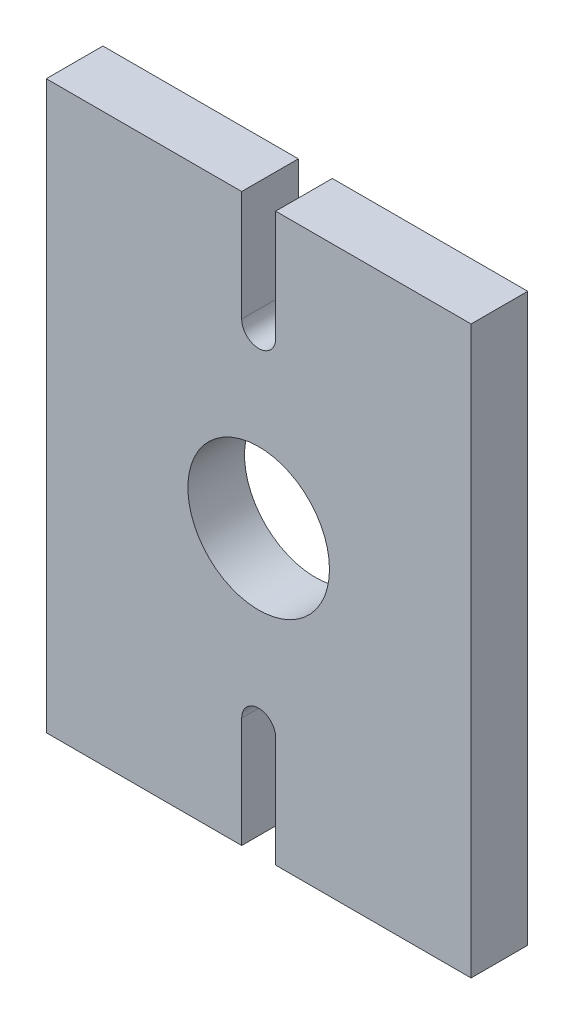
SolidWorks part; units mm, degrees
material "Q235"
ref_plane "Front Plane" through (0, 0, 0) normal (0, 0, 1) x (1, 0, 0)
ref_plane "Top Plane" through (0, 0, 0) normal (0, 1, 0) x (1, 0, 0)
ref_plane "Right Plane" through (0, 0, 0) normal (1, 0, 0) x (0, 0, -1)
sketch "Sketch1" plane through (0, 0, 0) normal (0, 0, 1) x (1, 0, 0)
  line L0 (75, 200) -> (75, 0) construction
  line L1 (0, 0) -> (69, 0)
  line L2 (0, 0) -> (0, 200)
  line L3 (0, 200) -> (69, 200)
  line L4 (150, 0) -> (150, 200)
  line L5 (0, 100) -> (150, 100) construction
  line L6 (69, 200) -> (69, 161)
  line L7 (81, 161) -> (81, 200)
  line L8 (69, 0) -> (69, 39)
  line L9 (81, 39) -> (81, 0)
  line L10 (81, 0) -> (150, 0)
  line L11 (81, 200) -> (150, 200)
  circle A0 centre (75, 100) radius 25
  arc A1 (69, 161) -> (81, 161) centre (75, 161) ccw
  arc A2 (69, 39) -> (81, 39) centre (75, 39) cw
  dimension "D3" = 50
  dimension "D6" = 39
  dimension "D7" = 39
  dimension "D10" = 75
  dimension "D1" = 200
  dimension "D2" = 150
  dimension "D4" = 6
  dimension "D5" = 12
  dimension "D8" = 6
  dimension "D9" = 12
extrude "Boss-Extrude1" add sketch "Sketch1" along normal blind 20
